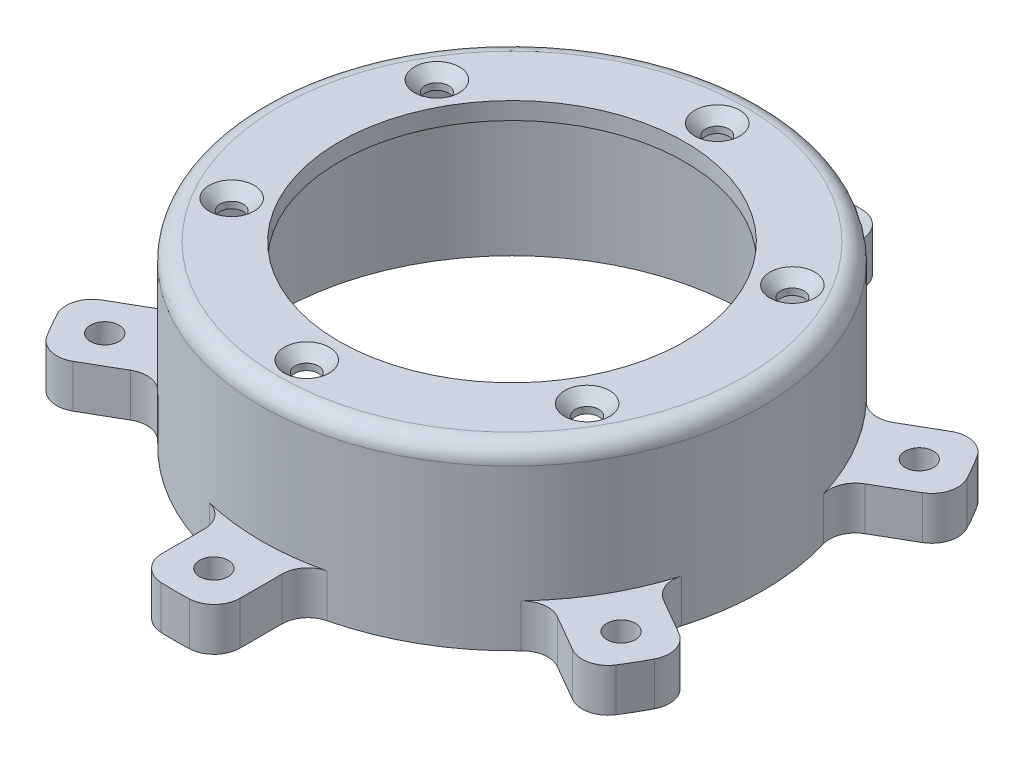
from build123d import *

# Parameters (mm, degrees)
SKETCH_1_R                   = 29
SKETCH_1_R_2                 = 20
SKETCH_1_R_3                 = 1.3
EXTRUDE_1_DEPTH              = 2
SKETCH_2_R                   = 29
SKETCH_2_R_2                 = 27
EXTRUDE_2_DEPTH              = 18.5
EXTRUDE_START                = -5
EXTRUDE_3_DEPTH              = 5
HOLE_WIZARD_M4_1_D           = 3.3
FILLET_1_R                   = 3
FILLET_2_R                   = 2
HOLE_WIZARD_M3_1_D           = 2.7
HOLE_WIZARD_M3_1_CSINK_D     = 5.2
HOLE_WIZARD_M3_1_CSINK_ANGLE = 90


with BuildPart() as part:
    # 草图1 → 凸台-拉伸1 (new body)
    with BuildSketch(Plane(origin=(0, 0, 0), x_dir=(1, 0, 0), z_dir=(0, 1, 0))):
        with Locations(Location((0, 0, 0), (0, 0, 270))):
            Circle(SKETCH_1_R)
        with Locations(Location((0, 0, 0), (0, 0, 270))):
            Circle(SKETCH_1_R_2, mode=Mode.SUBTRACT)
        with Locations(Location((0, 23.75, 0), (0, 0, 270))):
            Circle(SKETCH_1_R_3, mode=Mode.SUBTRACT)
        with Locations(Location((20.56810334, 11.875, 0), (0, 0, 270))):
            Circle(SKETCH_1_R_3, mode=Mode.SUBTRACT)
        with Locations(Location((20.56810334, -11.875, 0), (0, 0, 270))):
            Circle(SKETCH_1_R_3, mode=Mode.SUBTRACT)
        with Locations(Location((0, -23.75, 0), (0, 0, 270))):
            Circle(SKETCH_1_R_3, mode=Mode.SUBTRACT)
        with Locations(Location((-20.56810334, -11.875, 0), (0, 0, 270))):
            Circle(SKETCH_1_R_3, mode=Mode.SUBTRACT)
        with Locations(Location((-20.56810334, 11.875, 0), (0, 0, 270))):
            Circle(SKETCH_1_R_3, mode=Mode.SUBTRACT)
    extrude(amount=-EXTRUDE_1_DEPTH)

    # 草图2 → 凸台-拉伸2 (add)
    with BuildSketch(Plane.XZ.offset(2)):
        with Locations(Location((0, 0, 0), (0, 0, 90))):
            Circle(SKETCH_2_R)
        with Locations(Location((0, 0, 0), (0, 0, 270))):
            Circle(SKETCH_2_R_2, mode=Mode.SUBTRACT)
    extrude(amount=EXTRUDE_2_DEPTH)

    # 草图3 → 凸台-拉伸3 (add)
    with BuildSketch(Plane.XZ.offset(20.5).offset(EXTRUDE_START)):
        with BuildLine():
            Line((-4.5, 35.968736425), (-4.5, 28.648734702))
            ThreePointArc((-4.5, 28.648734702), (0, 29), (4.5, 28.648734702))
            Line((4.5, 28.648734702), (4.5, 35.968736425))
            ThreePointArc((4.5, 35.968736425), (3.665063509, 38.045392391), (1.625, 38.966131127))
            ThreePointArc((1.625, 38.966131127), (0, 39), (-1.625, 38.966131127))
            ThreePointArc((-1.625, 38.966131127), (-3.665063509, 38.045392391), (-4.5, 35.968736425))
        make_face()
        with BuildLine():
            Line((28.899839486, 21.881482529), (22.560532038, 18.221481668))
            ThreePointArc((22.560532038, 18.221481668), (25.11473671, 14.5), (27.060532038, 10.427253034))
            Line((27.060532038, 10.427253034), (33.399839486, 14.087253895))
            ThreePointArc((33.399839486, 14.087253895), (34.780808062, 15.84865809), (34.558159443, 18.075774282))
            ThreePointArc((34.558159443, 18.075774282), (33.774990748, 19.5), (32.933159443, 20.890356845))
            ThreePointArc((32.933159443, 20.890356845), (31.115744552, 22.196734301), (28.899839486, 21.881482529))
        make_face()
        with BuildLine():
            Line((33.399839486, -14.087253895), (27.060532038, -10.427253034))
            ThreePointArc((27.060532038, -10.427253034), (25.11473671, -14.5), (22.560532038, -18.221481668))
            Line((22.560532038, -18.221481668), (28.899839486, -21.881482529))
            ThreePointArc((28.899839486, -21.881482529), (31.115744552, -22.196734301), (32.933159443, -20.890356845))
            ThreePointArc((32.933159443, -20.890356845), (33.774990748, -19.5), (34.558159443, -18.075774282))
            ThreePointArc((34.558159443, -18.075774282), (34.780808062, -15.84865809), (33.399839486, -14.087253895))
        make_face()
        with BuildLine():
            Line((4.5, -35.968736425), (4.5, -28.648734702))
            ThreePointArc((4.5, -28.648734702), (0, -29), (-4.5, -28.648734702))
            Line((-4.5, -28.648734702), (-4.5, -35.968736425))
            ThreePointArc((-4.5, -35.968736425), (-3.665063509, -38.045392391), (-1.625, -38.966131127))
            ThreePointArc((-1.625, -38.966131127), (0, -39), (1.625, -38.966131127))
            ThreePointArc((1.625, -38.966131127), (3.665063509, -38.045392391), (4.5, -35.968736425))
        make_face()
        with BuildLine():
            Line((-28.899839486, -21.881482529), (-22.560532038, -18.221481668))
            ThreePointArc((-22.560532038, -18.221481668), (-25.11473671, -14.5), (-27.060532038, -10.427253034))
            Line((-27.060532038, -10.427253034), (-33.399839486, -14.087253895))
            ThreePointArc((-33.399839486, -14.087253895), (-34.780808062, -15.84865809), (-34.558159443, -18.075774282))
            ThreePointArc((-34.558159443, -18.075774282), (-33.774990748, -19.5), (-32.933159443, -20.890356845))
            ThreePointArc((-32.933159443, -20.890356845), (-31.115744552, -22.196734301), (-28.899839486, -21.881482529))
        make_face()
        with BuildLine():
            Line((-33.399839486, 14.087253895), (-27.060532038, 10.427253034))
            ThreePointArc((-27.060532038, 10.427253034), (-25.11473671, 14.5), (-22.560532038, 18.221481668))
            Line((-22.560532038, 18.221481668), (-28.899839486, 21.881482529))
            ThreePointArc((-28.899839486, 21.881482529), (-31.115744552, 22.196734301), (-32.933159443, 20.890356845))
            ThreePointArc((-32.933159443, 20.890356845), (-33.774990748, 19.5), (-34.558159443, 18.075774282))
            ThreePointArc((-34.558159443, 18.075774282), (-34.780808062, 15.84865809), (-33.399839486, 14.087253895))
        make_face()
    extrude(amount=EXTRUDE_3_DEPTH)

    # M4 螺纹孔1 (through all)
    with Locations(Plane.XZ.offset(20.5)):
        with Locations((-29.877876431, 17.25), (-29.877876431, -17.25), (0, -34.5), (29.877876431, -17.25), (29.877876431, 17.25), (0, 34.5)):
            Hole(HOLE_WIZARD_M4_1_D / 2)

    # 圆角1
    fillet_1_edges = [part.edges().sort_by_distance(p)[0] for p in [
        (-27.060532038, -18, -10.427253034),
        (-22.560532038, -18, -18.221481668),
        (-22.560532038, -18, 18.221481668),
        (-27.060532038, -18, 10.427253034),
        (4.5, -18, 28.648734702),
        (-4.5, -18, 28.648734702),
        (27.060532038, -18, 10.427253034),
        (22.560532038, -18, 18.221481668),
        (22.560532038, -18, -18.221481668),
        (27.060532038, -18, -10.427253034),
        (-4.5, -18, -28.648734702),
        (4.5, -18, -28.648734702),
    ]]
    fillet(fillet_1_edges, radius=FILLET_1_R)

    # 圆角2
    fillet_2_edges = [part.edges().sort_by_distance(p)[0] for p in [
        (0, 0, -29),
    ]]
    fillet(fillet_2_edges, radius=FILLET_2_R)

    # M3 内六角花形沉头螺钉的锥形沉头孔1 (through all)
    with Locations(Plane(origin=(0, 0, 0), x_dir=(1, 0, 0), z_dir=(0, 1, 0))):
        with Locations((0, 23.75), (20.56810334, 11.875), (20.56810334, -11.875), (0, -23.75), (-20.56810334, -11.875), (-20.56810334, 11.875)):
            CounterSinkHole(HOLE_WIZARD_M3_1_D / 2, HOLE_WIZARD_M3_1_CSINK_D / 2, counter_sink_angle=HOLE_WIZARD_M3_1_CSINK_ANGLE)


solid = part.part
